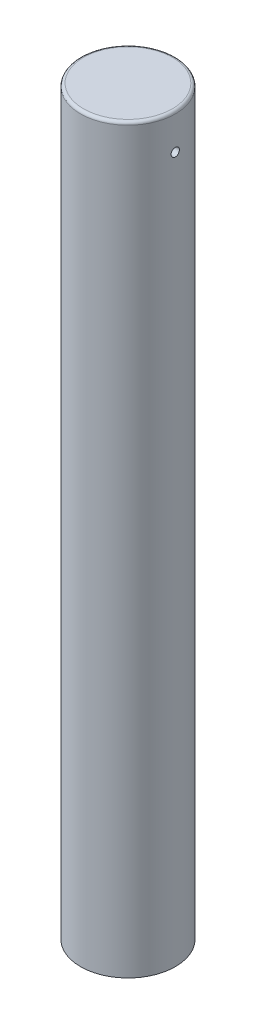
from build123d import *

# Parameters (mm, degrees)
CLEARANCE_HOLE_FOR_M1_61_D     = 1.8
CLEARANCE_HOLE_FOR_M1_61_DEPTH = 8
CLEARANCE_HOLE_FOR_M1_61_TIP   = 0.540774557


with BuildPart() as part:
    # Sketch1 → Revolution1 (revolve)
    with BuildSketch(Plane.XY, mode=Mode.PRIVATE) as revolution1_sk:
        with BuildLine():
            Line((0, -37.804295719), (-8, -37.804295719))
            Line((-8, -37.804295719), (-8, 86.695704281))
            ThreePointArc((-8, 86.695704281), (-7.853553391, 87.049257672), (-7.5, 87.195704281))
            Line((-7.5, 87.195704281), (0, 87.195704281))
            Line((0, 87.195704281), (0, -37.804295719))
        make_face()
    revolve(revolution1_sk.sketch.rotate(Axis((0, 38.205391481, 0), (0, -1, 0)), 270), axis=Axis((0, 38.205391481, 0), (0, -1, 0)))

    # Sketch2 → Cut-Revolve1 (revolve, cut)
    with BuildSketch(Plane.XY, mode=Mode.PRIVATE) as cut_revolve1_sk:
        with BuildLine():
            Line((8, 81.81366679), (6.5, 81.81366679))
            ThreePointArc((6.5, 81.81366679), (6.005025253, 81.608641537), (5.8, 81.11366679))
            Line((5.8, 81.11366679), (8, 81.11366679))
            Line((8, 81.11366679), (8, 81.81366679))
        make_face()
        with BuildLine():
            Line((-8, 81.11366679), (-8, 81.81366679))
            Line((-8, 81.81366679), (-6.5, 81.81366679))
            ThreePointArc((-6.5, 81.81366679), (-6.005025253, 81.608641537), (-5.8, 81.11366679))
            Line((-5.8, 81.11366679), (-8, 81.11366679))
        make_face()
    revolve(cut_revolve1_sk.sketch.rotate(Axis((8, 81.11366679, 0), (-1, 0, 0)), 90), axis=Axis((8, 81.11366679, 0), (-1, 0, 0)), mode=Mode.SUBTRACT)

    # Clearance hole for M1.61
    with Locations(Plane(origin=(0, -37.804295719, 0), x_dir=(-1, 0, 0), z_dir=(0, -1, 0))):
        with Locations((0, 0)):
            Hole(CLEARANCE_HOLE_FOR_M1_61_D / 2, depth=CLEARANCE_HOLE_FOR_M1_61_DEPTH)
            with Locations((0, 0, -(CLEARANCE_HOLE_FOR_M1_61_DEPTH + CLEARANCE_HOLE_FOR_M1_61_TIP / 2))):  # 118° drill point
                Cone(0, CLEARANCE_HOLE_FOR_M1_61_D / 2, CLEARANCE_HOLE_FOR_M1_61_TIP, mode=Mode.SUBTRACT)


solid = part.part
